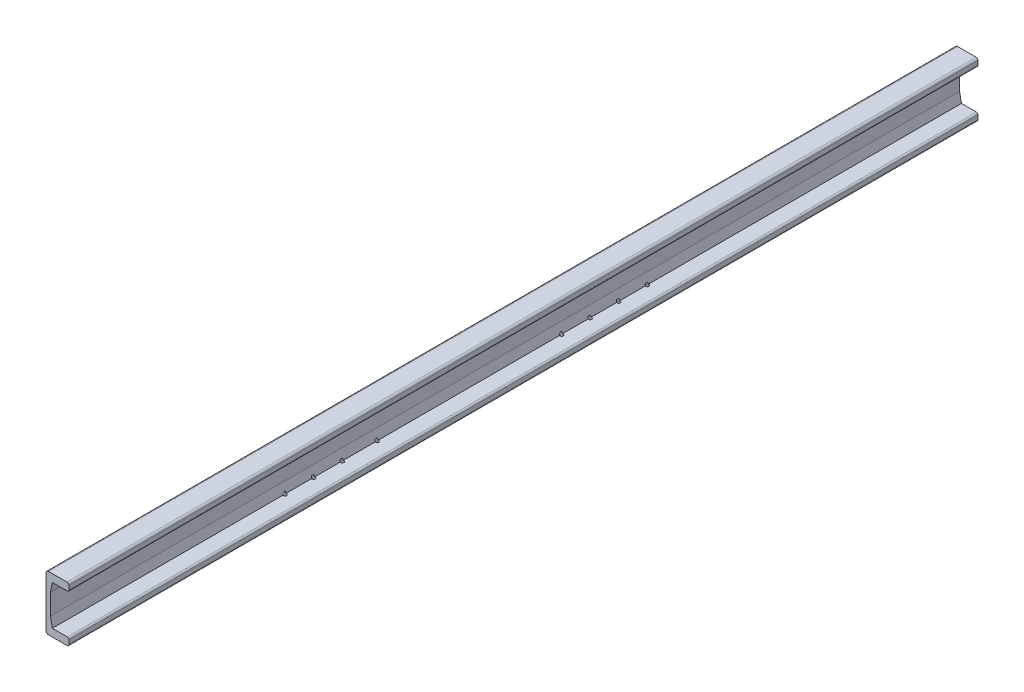
from build123d import *

# Parameters (mm, degrees)
BOSS_EXTRUDE1_DEPTH   = 1430
SKETCH2_R             = 2
CUT_EXTRUDE1_DEPTH    = 10
M6_TAPPED_HOLE1_D     = 5
M6_TAPPED_HOLE1_DEPTH = 15
M6_TAPPED_HOLE1_TIP   = 1.502151548


with BuildPart() as part:
    # Sketch1 → Boss-Extrude1 (new body)
    with BuildSketch(Plane.XY):
        with BuildLine():
            Line((-3, 0), (-32, 0))
            ThreePointArc((-32, 0), (-34.828427125, -1.171572875), (-36, -4))
            Line((-36, -4), (-36, -82.5))
            ThreePointArc((-36, -82.5), (-34.828427125, -85.328427125), (-32, -86.5))
            Line((-32, -86.5), (-3, -86.5))
            ThreePointArc((-3, -86.5), (-0.878679656, -85.621320344), (0, -83.5))
            Line((0, -83.5), (0, -77))
            ThreePointArc((0, -77), (-0.732233047, -75.232233047), (-2.5, -74.5))
            Line((-2.5, -74.5), (-26, -74.5))
            Line((-26, -74.5), (-29, -59.5))
            Line((-29, -59.5), (-29, -27))
            Line((-29, -27), (-26, -12))
            Line((-26, -12), (-2.5, -12))
            ThreePointArc((-2.5, -12), (-0.732233047, -11.267766953), (0, -9.5))
            Line((0, -9.5), (0, -3))
            ThreePointArc((0, -3), (-0.878679656, -0.878679656), (-3, 0))
        make_face()
    extrude(amount=BOSS_EXTRUDE1_DEPTH)

    # Sketch2 → Cut-Extrude1 (cut)
    with BuildSketch(Plane.XZ.offset(86.5)):
        with Locations(Location((-25, 495, 0), (0, 0, 270))):
            Circle(SKETCH2_R)
        with Locations(Location((-25, 540, 0), (0, 0, 270))):
            Circle(SKETCH2_R)
        with Locations(Location((-25, 975, 0), (0, 0, 270))):
            Circle(SKETCH2_R)
        with Locations(Location((-25, 585, 0), (0, 0, 270))):
            Circle(SKETCH2_R)
        with Locations(Location((-25, 630, 0), (0, 0, 270))):
            Circle(SKETCH2_R)
        with Locations(Location((-25, 1065, 0), (0, 0, 270))):
            Circle(SKETCH2_R)
        with Locations(Location((-25, 920, 0), (0, 0, 270))):
            Circle(SKETCH2_R)
        with Locations(Location((-25, 1020, 0), (0, 0, 270))):
            Circle(SKETCH2_R)
    extrude(amount=-CUT_EXTRUDE1_DEPTH, mode=Mode.SUBTRACT)

    # M6 Tapped Hole1
    with Locations(Plane(origin=(0, -86.5, 0), x_dir=(-1, 0, 0), z_dir=(0, -1, 0))):
        with Locations((25, -630), (25, -585), (25, -540), (25, -495), (25, -920), (25, -975), (25, -1020), (25, -1065)):
            Hole(M6_TAPPED_HOLE1_D / 2, depth=M6_TAPPED_HOLE1_DEPTH)
            with Locations((0, 0, -(M6_TAPPED_HOLE1_DEPTH + M6_TAPPED_HOLE1_TIP / 2))):  # 118° drill point
                Cone(0, M6_TAPPED_HOLE1_D / 2, M6_TAPPED_HOLE1_TIP, mode=Mode.SUBTRACT)


solid = part.part
